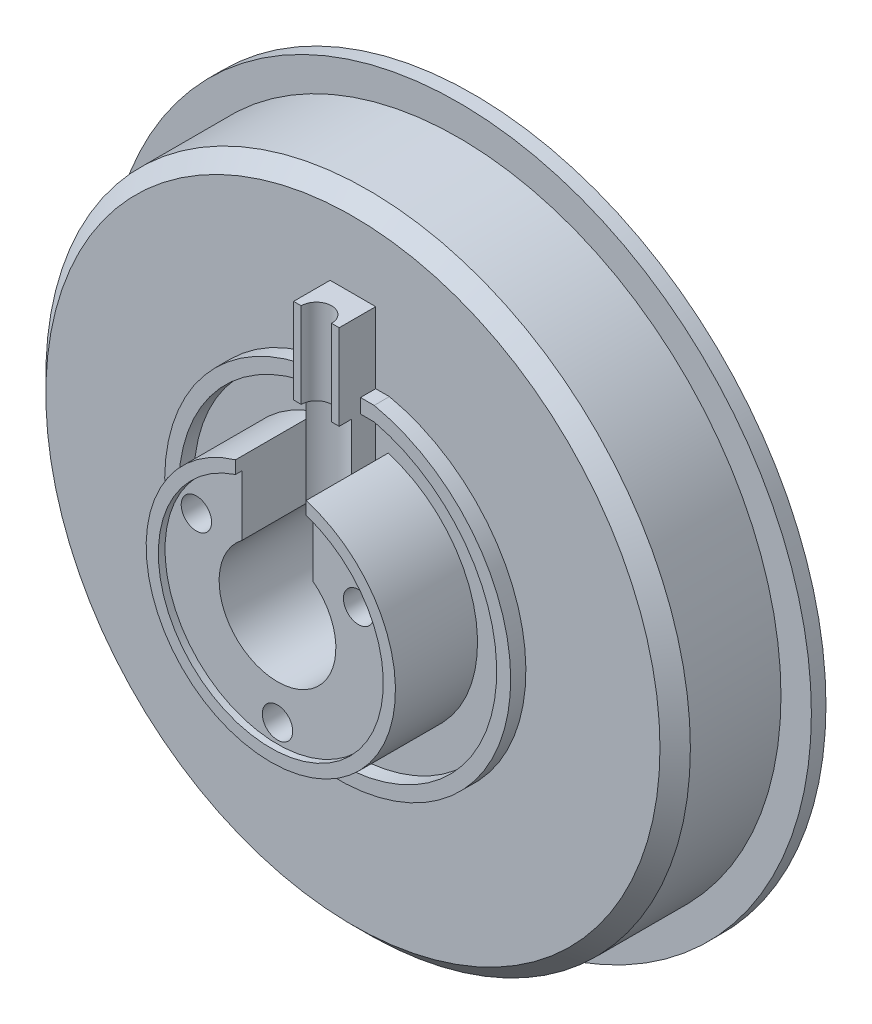
SolidWorks part; units mm, degrees
material "ABS"
ref_plane "前视基准面" through (0, 0, 0) normal (0, 0, 1) x (1, 0, 0)
ref_plane "上视基准面" through (0, 0, 0) normal (0, 1, 0) x (1, 0, 0)
ref_plane "右视基准面" through (0, 0, 0) normal (1, 0, 0) x (0, 0, -1)
sketch "草图1" plane through (0, 0, 0) normal (0, 0, 1) x (1, 0, 0)
  circle A0 centre (0, 0) radius 58
extrude "凸台-拉伸1" add sketch "草图1" along normal blind 2.4
sketch "草图2" plane through (0, 0, 2.4) normal (0, 0, 1) x (1, 0, 0)
  circle A0 centre (0, 0) radius 53
  dimension "D1" = 106
extrude "凸台-拉伸2" add sketch "草图2" along normal blind 17.4
chamfer "倒角1" distance 2.5 angle 45 1 edges at (53, 0, 19.8)
sketch "草图3" plane through (0, 0, 19.8) normal (0, 0, 1) x (1, 0, 0)
  circle A0 centre (0, 0) radius 20.5
extrude "凸台-拉伸3" add sketch "草图3" along normal blind 13.5
sketch "草图4" plane through (0, 0, 33.3) normal (0, 0, 1) x (1, 0, 0)
  circle A0 centre (0, 0) radius 18.5
extrude "切除-拉伸1" cut sketch "草图4" against normal blind 1.1
sketch "草图5" plane through (0, 0, 32.2) normal (0, 0, 1) x (1, 0, 0)
  circle A0 centre (0, 0) radius 15.4 construction
  circle A1 centre (0, -15.4) radius 2.5
  circle A2 centre (-13.3368, 7.7) radius 2.5
  circle A3 centre (13.3368, 7.7) radius 2.5
  point P11 (0, 0)
  dimension "D1" = 3
extrude "切除-拉伸2" cut sketch "草图5" against normal blind 320
sketch "草图6" plane through (0, 0, 0) normal (0, 0, -1) x (-1, 0, 0)
  circle A0 centre (0, 0) radius 50.5
extrude "切除-拉伸3" cut sketch "草图6" against normal blind 16.5
sketch "草图7" plane through (0, 0, 16.5) normal (0, 0, -1) x (-1, 0, 0)
  line L0 (-11.7085, 0.9864) -> (-17.9252, 4.5756)
  line L1 (0, 60.1572) -> (0, -61.3376) construction
  line L2 (5, -10.6331) -> (5, -17.8115)
  line L3 (-5, -10.6331) -> (-5, -17.8115)
  line L4 (-7, 9.815) -> (-12.9252, 13.2359)
  line L5 (7, 9.815) -> (12.9252, 13.2359)
  line L6 (11.7085, 0.9864) -> (17.9252, 4.5756)
  line L7 (7, 9.815) -> (7, 17.1245)
  line L8 (-7, 9.815) -> (-7, 17.1245)
  arc A0 (5, -17.8115) -> (17.9252, 4.5756) centre (0, 0) ccw
  arc A1 (5, -10.6331) -> (11.7085, 0.9864) centre (0, 0) ccw
  arc A3 (12.9252, 13.2359) -> (7, 17.1245) centre (0, 0) ccw
  arc A4 (-11.7085, 0.9864) -> (-5, -10.6331) centre (0, 0) ccw
  arc A5 (-17.9252, 4.5756) -> (-5, -17.8115) centre (0, 0) ccw
  arc A7 (-7, 17.1245) -> (-12.9252, 13.2359) centre (0, 0) ccw
  point P21 (0, 0)
  dimension "D1" = 10
  dimension "D2" = 37
  dimension "D3" = 23.5
  dimension "D5" = 14
  dimension "D4" = 3
extrude "切除-拉伸5" cut sketch "草图7" against normal blind 13
sketch "草图8" plane through (0, 0, 19.8) normal (0, 0, 1) x (1, 0, 0)
  line L0 (0, -64.4576) -> (0, 62.0606) construction
  line L1 (-6, 27.8101) -> (6, 27.8101)
  line L2 (-6, 25.4524) -> (6, 25.4524)
  arc A0 (-6, 27.8101) -> (6, 27.8101) centre (0, 0) ccw
  arc A1 (-6, 25.4524) -> (6, 25.4524) centre (0, 0) ccw
  dimension "D1" = 56.9
  dimension "D2" = 52.3
  dimension "D3" = 12
  dimension "D4" = 6
  dimension "D5" = 12
extrude "凸台-拉伸4" add sketch "草图8" along normal blind 2.5
sketch "草图9" plane through (0, 0, 33.3) normal (0, 0, 1) x (1, 0, 0)
  line L0 (0, 0) -> (0, 29.0569) construction
  line L1 (-5.8, 0) -> (5.8, 0)
  line L2 (-5.8, 0) -> (-5.8, 21.8861)
  line L3 (-5.8, 21.8861) -> (5.8, 21.8861)
  line L4 (5.8, 0) -> (5.8, 21.8861)
  line L5 (-5.8, 0) -> (5.8, 21.8861) construction
  line L6 (-5.8, 21.8861) -> (5.8, 0) construction
  point P0 (0, 10.943)
  dimension "D1" = 11.6
extrude "切除-拉伸6" cut sketch "草图9" against normal up to surface (13.5 mm away) up to face at (0, -0.3488, 19.8)
sketch "草图11" plane through (0, 0, 0) normal (0, 1, 0) x (1, 0, 0)
  line L0 (0, 4.4501) -> (0, -37.4548) construction
  line L1 (-3.75, -19.8) -> (3.75, -19.8)
  line L2 (6, -19.8) -> (-6, -19.8) construction
  line L3 (3.75, -19.8) -> (3.75, -23.8)
  line L4 (-3.75, -19.8) -> (-3.75, -23.8)
  line L5 (2.2004, -21.8) -> (-2.0502, -21.8) construction
  arc A0 (3.75, -23.8) -> (-3.75, -23.8) centre (0, -26.3156) ccw
  point P10 (0, -19.8)
  dimension "D1" = 3.75
  dimension "D2" = 4
  dimension "D3" = 2
extrude "凸台-拉伸5" add sketch "草图11" along normal blind 39.5
sketch "草图12" plane through (0, 39.5, 0) normal (0, 1, 0) x (1, 0, 0)
  line L0 (-3.75, -23.8) -> (-3.75, -25.8)
  line L1 (-3.75, -25.8) -> (-2.5, -25.8)
  line L2 (0, -35.5866) -> (0, -28.3) construction
  line L3 (3.75, -25.8) -> (2.5, -25.8)
  line L4 (3.75, -23.8) -> (3.75, -25.8)
  line L5 (0, -23.3) -> (0, -20.7522) construction
  arc A0 (2.5, -25.8) -> (-2.5, -25.8) centre (0, -25.8) ccw
  arc A1 (3.75, -23.8) -> (-3.75, -23.8) centre (0, -26.3156) ccw construction
  arc A2 (3.75, -23.8) -> (-3.75, -23.8) centre (0, -26.3156) ccw
  dimension "D1" = 2
  dimension "D2" = 1.25
extrude "凸台-拉伸6" add sketch "草图12" against normal up to surface (14.0476 mm away) up to face at (0, 25.4524, 22.05)
sketch "草图10" plane through (0, 0, 32.2) normal (0, 0, 1) x (1, 0, 0)
  circle A0 centre (0, 0) radius 9.6
extrude "切除-拉伸7" cut sketch "草图10" against normal up to next
